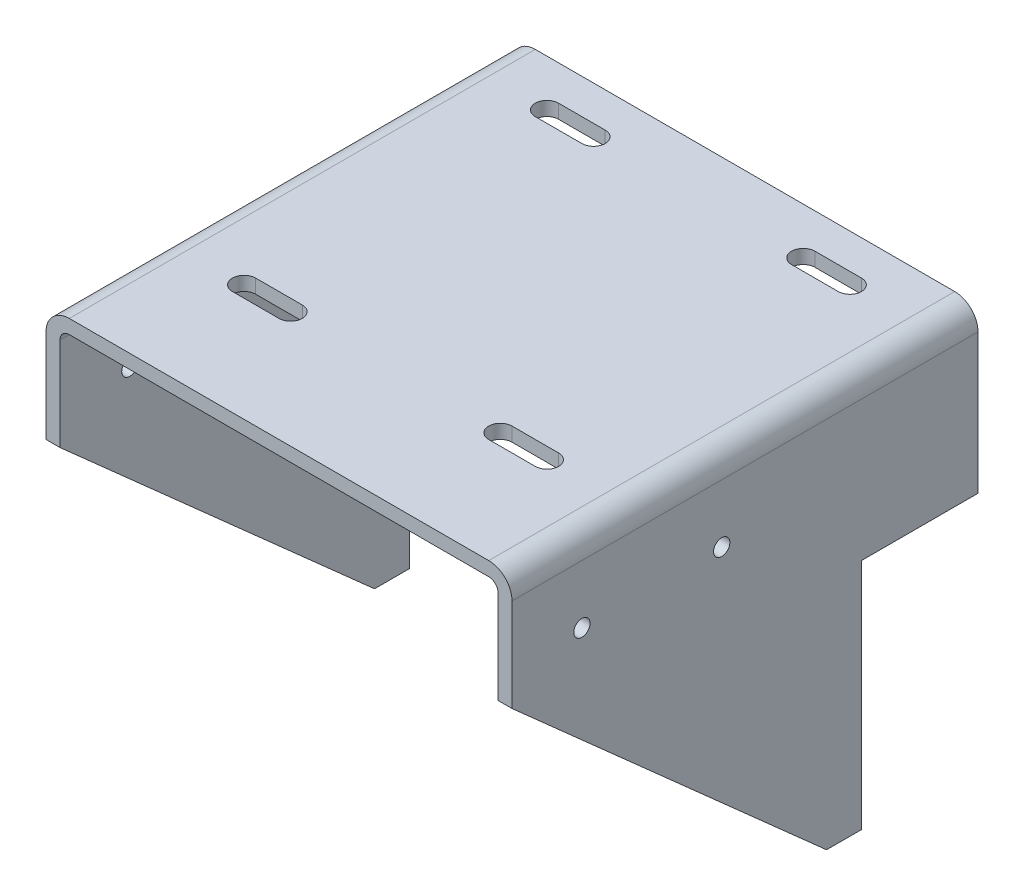
SolidWorks part; units mm, degrees
material "1023 Carbon Steel Plate (SS)"
ref_plane "Front Plane" through (0, 0, 0) normal (0, 0, 1) x (1, 0, 0)
ref_plane "Top Plane" through (0, 0, 0) normal (0, 1, 0) x (1, 0, 0)
ref_plane "Right Plane" through (0, 0, 0) normal (1, 0, 0) x (0, 0, -1)
sketch "Sketch1" plane through (0, 0, 0) normal (0, 0, 1) x (1, 0, 0)
  line L0 (0, 0) -> (0, 160)
  line L1 (10, 170) -> (190, 170)
  line L2 (200, 160) -> (200, 0)
  line L3 (6, 0) -> (6, 160)
  line L4 (10, 164) -> (190, 164)
  line L5 (194, 160) -> (194, 0)
  line L6 (6, 0) -> (0, 0)
  line L7 (200, 0) -> (194, 0)
  arc A0 (190, 170) -> (200, 160) centre (190, 160) cw
  arc A1 (0, 160) -> (10, 170) centre (10, 160) cw
  arc A2 (6, 160) -> (10, 164) centre (10, 160) cw
  arc A3 (190, 164) -> (194, 160) centre (190, 160) cw
  point P7 (200, 170)
  point P10 (0, 170)
  dimension "D3" = 10
  dimension "D1" = 170
  dimension "D2" = 200
  dimension "D4" = 6
extrude "Boss-Extrude2" add sketch "Sketch1" along normal blind 200 contours L7 L5 A3 L4 A2 L3 L6 L0 A1 L1 A0 L2
sketch "Sketch2" plane through (200, 0, 0) normal (1, 0, 0) x (0, 0, -1)
  line L0 (-200, 120) -> (-65, 0)
  line L1 (-200, 160) -> (-200, 0) construction
  line L2 (-200, 0) -> (0, 0) construction
  line L3 (-65, 0) -> (-50, 0)
  line L4 (-50, 0) -> (-50, 100)
  line L5 (-50, 100) -> (0, 100)
  line L6 (0, 160) -> (0, 0) construction
  line L7 (0, 100) -> (0, -9.1627)
  line L8 (0, -9.1627) -> (-225.1497, -7.961)
  line L9 (-225.1497, -7.961) -> (-227.0381, 77.7684)
  line L10 (-227.0381, 77.7684) -> (-200, 120)
  dimension "D1" = 15
  dimension "D2" = 50
  dimension "D3" = 100
  dimension "D4" = 120
extrude "Cut-Extrude1" cut sketch "Sketch2" against normal blind 200
sketch "Sketch3" plane through (200, 0, 0) normal (1, 0, 0) x (0, 0, -1)
  line L0 (-200, 160) -> (-200, 120) construction
  line L1 (-200, 170) -> (0, 170) construction
  circle A0 centre (-170, 135) radius 3.5
  circle A1 centre (-110, 135) radius 3.5
  dimension "D2" = 7
  dimension "D3" = 30
  dimension "D1" = 60
  dimension "D4" = 35
extrude "Cut-Extrude2" cut sketch "Sketch3" against normal blind 200
sketch "Sketch4" plane through (0, 170, 0) normal (0, 1, 0) x (1, 0, 0)
  line L0 (165, -20) -> (145, -20) construction
  line L3 (165, -25) -> (145, -25)
  line L6 (165, -15) -> (145, -15)
  line L9 (165, -150) -> (145, -150) construction
  line L12 (10, 0) -> (190, 0) construction
  line L13 (165, -155) -> (145, -155)
  line L14 (200, -200) -> (200, 0) construction
  line L15 (165, -145) -> (145, -145)
  line L16 (55, -20) -> (35, -20) construction
  line L17 (55, -25) -> (35, -25)
  line L18 (55, -15) -> (35, -15)
  line L19 (55, -150) -> (35, -150) construction
  line L20 (55, -155) -> (35, -155)
  line L21 (55, -145) -> (35, -145)
  arc A8 (165, -25) -> (165, -15) centre (165, -20) ccw
  arc A9 (145, -15) -> (145, -25) centre (145, -20) ccw
  arc A10 (165, -155) -> (165, -145) centre (165, -150) ccw
  arc A11 (145, -145) -> (145, -155) centre (145, -150) ccw
  arc A12 (55, -25) -> (55, -15) centre (55, -20) ccw
  arc A13 (35, -15) -> (35, -25) centre (35, -20) ccw
  arc A14 (55, -155) -> (55, -145) centre (55, -150) ccw
  arc A15 (35, -145) -> (35, -155) centre (35, -150) ccw
  point P2 (155, -20)
  point P7 (155, -150)
  point P14 (45, -20)
  point P21 (45, -150)
  dimension "D2" = 20
  dimension "D5" = 90
  dimension "D6" = 35
  dimension "D4" = 5
  dimension "D1" = 130
  dimension "D3" = 20
extrude "Cut-Extrude3" cut sketch "Sketch4" against normal blind 10
